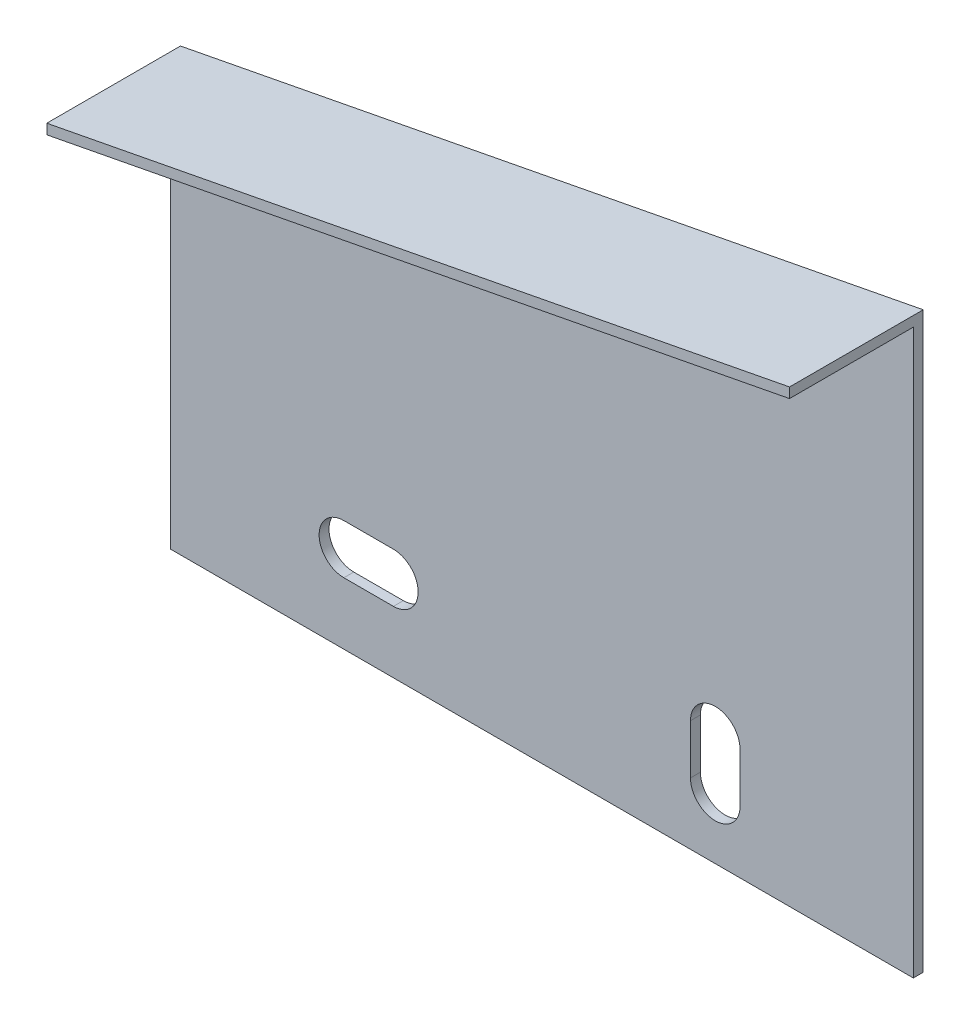
from build123d import *

# Parameters (mm, degrees)
BOSS_EXTRUDE1_DEPTH = 4
BOSS_EXTRUDE2_DEPTH = 50


with BuildPart() as part:
    # Sketch1 → Boss-Extrude1 (new body)
    with BuildSketch(Plane.XY):
        Polygon((0, 174), (300, 231.742517927), (300, 0), (0, 0), align=None)
        with BuildLine():
            Line((70, 45), (90, 45))
            ThreePointArc((90, 45), (100, 35), (90, 25))
            Line((90, 25), (70, 25))
            ThreePointArc((70, 25), (60, 35), (70, 45))
        make_face(mode=Mode.SUBTRACT)
        with BuildLine():
            Line((230, 45), (230, 25))
            ThreePointArc((230, 25), (220, 15), (210, 25))
            Line((210, 25), (210, 45))
            ThreePointArc((210, 45), (220, 55), (230, 45))
        make_face(mode=Mode.SUBTRACT)
    extrude(amount=BOSS_EXTRUDE1_DEPTH)

    # Sketch2 → Boss-Extrude2 (add)
    with BuildSketch(Plane.XY.offset(4)):
        Polygon((21.16336267, 174), (300, 227.669098433), (300, 231.742517927), (0, 174), (0, 169.926580506), align=None)
    extrude(amount=BOSS_EXTRUDE2_DEPTH)


solid = part.part
